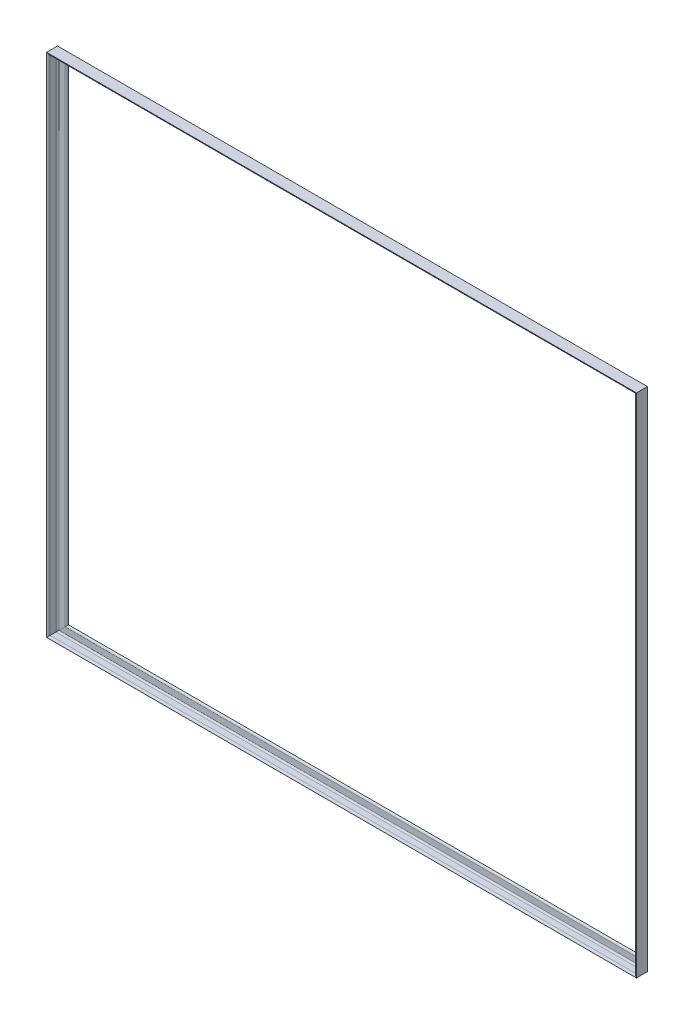
from build123d import *

# Parameters (mm, degrees)
ANGLE_IRON_CONFIGURED_25_X_25_X_4_1_DEPTH      = 1194.355339059
ANGLE_IRON_CONFIGURED_25_X_25_X_4_1_DEPTH_BACK = 36.355339059
ANGLE_IRON_CONFIGURED_25_X_25_X_4_1_2_DEPTH    = 1420.710678119
ANGLE_IRON_CONFIGURED_25_X_25_X_4_1_3_DEPTH    = 1230.710678119
ANGLE_IRON_CONFIGURED_25_X_25_X_4_1_4_DEPTH    = 1420.710678119


with BuildPart() as part:
    # Sketch1 → Angle iron - configured 25 X 25 X 4(1) (new, two sides: drawn at the far end of the back side and taken through both)
    with BuildSketch(Plane(origin=(-674, 579, 0), x_dir=(1, 0, 0), z_dir=(0, -1, 0)).offset(-ANGLE_IRON_CONFIGURED_25_X_25_X_4_1_DEPTH_BACK)):
        with BuildLine():
            Line((0, 0), (0, 25))
            ThreePointArc((0, 25), (2.828427125, 23.828427125), (4, 21))
            Line((4, 21), (4, 7.5))
            ThreePointArc((4, 7.5), (5.025126266, 5.025126266), (7.5, 4))
            Line((7.5, 4), (21, 4))
            ThreePointArc((21, 4), (23.828427125, 2.828427125), (25, 0))
            Line((25, 0), (0, 0))
        make_face()
    extrude(amount=ANGLE_IRON_CONFIGURED_25_X_25_X_4_1_DEPTH + ANGLE_IRON_CONFIGURED_25_X_25_X_4_1_DEPTH_BACK)

    # Angle iron - configured 25 X 25 X 4(1) mi
    split(bisect_by=Plane(origin=(-674, 579, 0), x_dir=(0.707106781, -0.707106781, 0), z_dir=(-0.707106781, -0.707106781, 0)), keep=Keep.TOP)

    # Angle iron - configured 25 X 25 X 4_ 2
    split(bisect_by=Plane(origin=(-674, -579, 0), x_dir=(-0.707106781, -0.707106781, 0), z_dir=(-0.707106781, 0.707106781, 0)), keep=Keep.TOP)


with BuildPart() as body_2:
    # Sketch1 on segment 2 (carried to segment 2) → Angle iron - configured 25 X 25 X 4_1 2 (new body)
    with BuildSketch(Plane(origin=(-710.355339059, -579, 0), x_dir=(0, 1, 0), z_dir=(1, 0, 0))):
        with BuildLine():
            Line((0, 0), (0, 25))
            ThreePointArc((0, 25), (2.828427125, 23.828427125), (4, 21))
            Line((4, 21), (4, 7.5))
            ThreePointArc((4, 7.5), (5.025126266, 5.025126266), (7.5, 4))
            Line((7.5, 4), (21, 4))
            ThreePointArc((21, 4), (23.828427125, 2.828427125), (25, 0))
            Line((25, 0), (0, 0))
        make_face()
    extrude(amount=ANGLE_IRON_CONFIGURED_25_X_25_X_4_1_2_DEPTH)

    # Angle iron - configured 25 X 25 X 4_ 3
    split(bisect_by=Plane(origin=(-674, -579, 0), x_dir=(0.707106781, 0.707106781, 0), z_dir=(0.707106781, -0.707106781, 0)), keep=Keep.TOP)

    # Angle iron - configured 25 X 25 X 4_ 4
    split(bisect_by=Plane(origin=(674, -579, 0), x_dir=(0.707106781, -0.707106781, 0), z_dir=(-0.707106781, -0.707106781, 0)), keep=Keep.TOP)


with BuildPart() as body_3:
    # Sketch1 on segment 3 (carried to segment 3) → Angle iron - configured 25 X 25 X 4_1 3 (new body)
    with BuildSketch(Plane(origin=(674, -615.355339059, 0), x_dir=(-1, 0, 0), z_dir=(0, 1, 0))):
        with BuildLine():
            Line((0, 0), (0, 25))
            ThreePointArc((0, 25), (2.828427125, 23.828427125), (4, 21))
            Line((4, 21), (4, 7.5))
            ThreePointArc((4, 7.5), (5.025126266, 5.025126266), (7.5, 4))
            Line((7.5, 4), (21, 4))
            ThreePointArc((21, 4), (23.828427125, 2.828427125), (25, 0))
            Line((25, 0), (0, 0))
        make_face()
    extrude(amount=ANGLE_IRON_CONFIGURED_25_X_25_X_4_1_3_DEPTH)

    # Angle iron - configured 25 X 25 X 4_ 5
    split(bisect_by=Plane(origin=(674, 579, 0), x_dir=(0.707106781, 0.707106781, 0), z_dir=(0.707106781, -0.707106781, 0)), keep=Keep.TOP)

    # Angle iron - configured 25 X 25 X 4_ 6
    split(bisect_by=Plane(origin=(674, -579, 0), x_dir=(-0.707106781, 0.707106781, 0), z_dir=(0.707106781, 0.707106781, 0)), keep=Keep.TOP)


with BuildPart() as body_4:
    # Sketch1 on segment 4 (carried to segment 4) → Angle iron - configured 25 X 25 X 4_1 4 (new body)
    with BuildSketch(Plane(origin=(710.355339059, 579, 0), x_dir=(0, -1, 0), z_dir=(-1, 0, 0))):
        with BuildLine():
            Line((0, 0), (0, 25))
            ThreePointArc((0, 25), (2.828427125, 23.828427125), (4, 21))
            Line((4, 21), (4, 7.5))
            ThreePointArc((4, 7.5), (5.025126266, 5.025126266), (7.5, 4))
            Line((7.5, 4), (21, 4))
            ThreePointArc((21, 4), (23.828427125, 2.828427125), (25, 0))
            Line((25, 0), (0, 0))
        make_face()
    extrude(amount=ANGLE_IRON_CONFIGURED_25_X_25_X_4_1_4_DEPTH)

    # Angle iron - configured 25 X 25 X 4_ 7
    split(bisect_by=Plane(origin=(-674, 579, 0), x_dir=(-0.707106781, 0.707106781, 0), z_dir=(0.707106781, 0.707106781, 0)), keep=Keep.TOP)

    # Angle iron - configured 25 X 25 X 4_ 8
    split(bisect_by=Plane(origin=(674, 579, 0), x_dir=(-0.707106781, -0.707106781, 0), z_dir=(-0.707106781, 0.707106781, 0)), keep=Keep.TOP)


solid = Compound([part.part, body_2.part, body_3.part, body_4.part])
